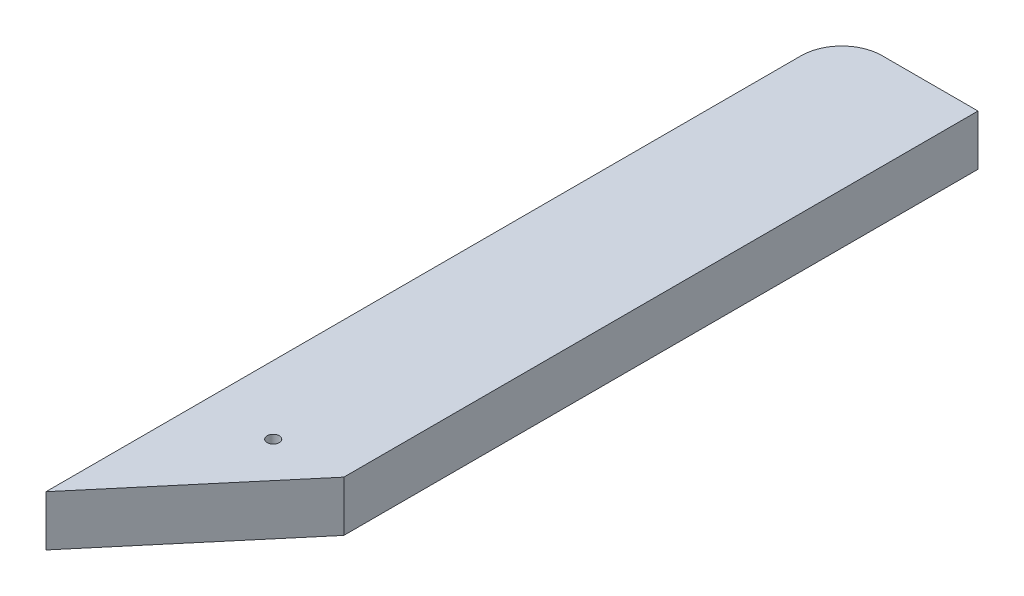
from build123d import *

# Parameters (mm, degrees)
SKETCH1_R           = 3
BOSS_EXTRUDE1_DEPTH = 25
FILLET1_R           = 20


with BuildPart() as part:
    # Sketch1 → Boss-Extrude1 (new body)
    with BuildSketch(Plane(origin=(0, 0, 0), x_dir=(1, 0, 0), z_dir=(0, 1, 0))):
        Polygon((67.5, 0), (0, 0), (0, -394.016321232), (67.5, -314.016321232), align=None)
        with Locations(Location((33.75, -315.248874166, 0), (0, 0, 270))):
            Circle(SKETCH1_R, mode=Mode.SUBTRACT)
    extrude(amount=BOSS_EXTRUDE1_DEPTH)

    # Fillet1
    fillet1_edges = [part.edges().sort_by_distance(p)[0] for p in [
        (0, 12.5, 0),
    ]]
    fillet(fillet1_edges, radius=FILLET1_R)


solid = part.part
